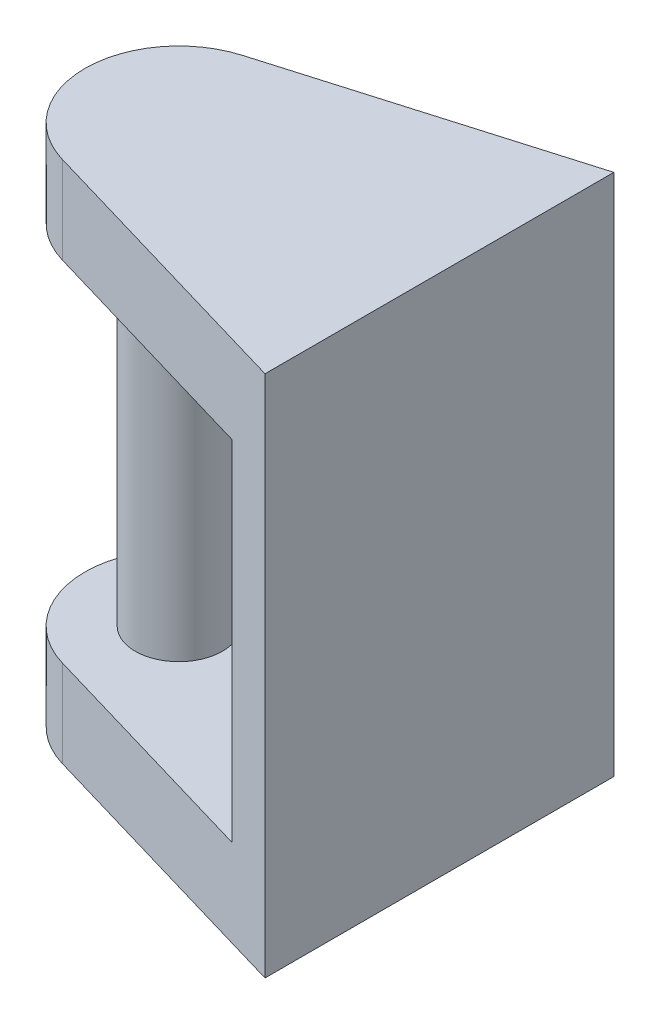
SolidWorks part; units mm, degrees
ref_plane "Front Plane" through (0, 0, 0) normal (0, 0, 1) x (1, 0, 0)
ref_plane "Top Plane" through (0, 0, 0) normal (0, 1, 0) x (1, 0, 0)
ref_plane "Right Plane" through (0, 0, 0) normal (1, 0, 0) x (0, 0, -1)
sketch "Sketch1" plane through (0, 0, 0) normal (0, 1, 0) x (1, 0, 0)
  line L0 (0, 0) -> (0, -40)
  line L1 (0, 0) -> (-32.9168, -9.6735)
  line L2 (0, -40) -> (-32.9168, -30.3265)
  line L3 (0, -20) -> (-54.9892, -20) construction
  arc A1 (-32.9168, -30.3265) -> (-32.9168, -9.6735) centre (-29.8821, -20) cw
  dimension "D1" = 40
extrude "Boss-Extrude1" add sketch "Sketch1" along normal blind 60
ref_plane "Plane1" through (0, 10, 0) normal (0, -1, 0) x (-1, 0, 0)
sketch "Sketch2" plane through (0, 10, 0) normal (0, -1, 0) x (-1, 0, 0)
  line L0 (5.3815, -1.5815) -> (5.3815, -38.4185)
  line L3 (0, 0) -> (0, -40)
  line L4 (0, -40) -> (32.9168, -30.3265)
  line L5 (32.9168, -9.6735) -> (0, 0)
  line L7 (5.3815, -38.4185) -> (32.9168, -30.3265)
  line L8 (32.9168, -9.6735) -> (5.3815, -1.5815)
  arc A1 (32.9168, -30.3265) -> (32.9168, -9.6735) centre (29.8821, -20) ccw
  arc A2 (32.9168, -30.3265) -> (32.9168, -9.6735) centre (29.8821, -20) ccw
  dimension "D1" = 0
extrude "Cut-Extrude1" cut sketch "Sketch2" against normal blind 40
sketch "Sketch3" plane through (0, 10, 0) normal (0, -1, 0) x (-1, 0, 0)
  circle A0 centre (29.8821, -20) radius 5
  dimension "D1" = 10
extrude "Boss-Extrude2" add sketch "Sketch3" against normal up to next
